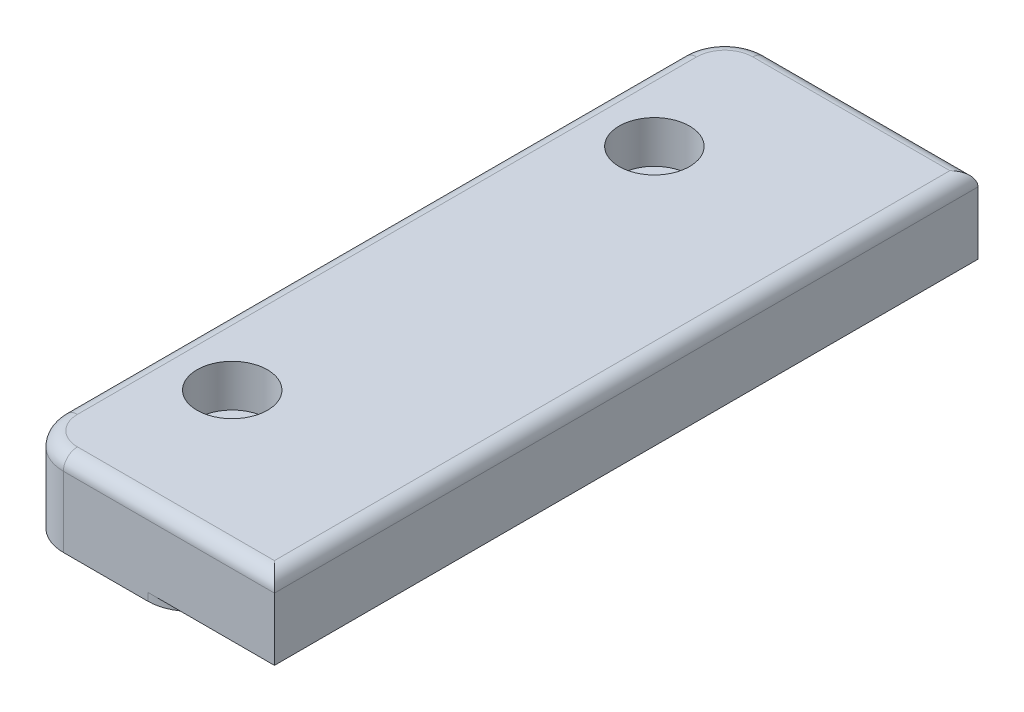
from build123d import *

# Parameters (mm, degrees)
BOSS_EXTRUDE1_DEPTH = 50
FILLET1_R           = 3
SKETCH3_R           = 2.5
CUT_EXTRUDE1_DEPTH  = 3
SKETCH4_R           = 1.5
CUT_EXTRUDE2_DEPTH  = 52.816130281
SKETCH5_R           = 1.5
CUT_EXTRUDE3_DEPTH  = 52.816130281
FILLET5_R           = 3
FILLET6_R           = 3
FILLET7_R           = 1


with BuildPart() as part:
    # Sketch1 → Boss-Extrude1 (new body)
    with BuildSketch(Plane.XY):
        Polygon((-4.736842105, 0), (-4.736842105, 6), (13.263157895, 6), (13.263157895, 0.55), (7.263157895, 0.55), (7.263157895, 0), align=None)
    extrude(amount=BOSS_EXTRUDE1_DEPTH)

    # Fillet1
    fillet1_edges = [part.edges().sort_by_distance(p)[0] for p in [
        (7.263157895, 0.275, 50),
    ]]
    fillet(fillet1_edges, radius=FILLET1_R)

    # Sketch3 → Cut-Extrude1 (cut)
    with BuildSketch(Plane(origin=(0, 6, 0), x_dir=(1, 0, 0), z_dir=(0, 1, 0))):
        with Locations(Location((0.263157895, -10, 0), (0, 0, 180))):
            Circle(SKETCH3_R)
        with Locations(Location((0.263157895, -40, 0), (0, 0, 180))):
            Circle(SKETCH3_R)
    extrude(amount=-CUT_EXTRUDE1_DEPTH, mode=Mode.SUBTRACT)

    # Sketch4 → Cut-Extrude2 (cut, through all)
    with BuildSketch(Plane(origin=(0, 3, 0), x_dir=(1, 0, 0), z_dir=(0, 1, 0))):
        with Locations(Location((0.263157895, -40, 0), (0, 0, 180))):
            Circle(SKETCH4_R)
    extrude(amount=-CUT_EXTRUDE2_DEPTH, mode=Mode.SUBTRACT)

    # Sketch5 → Cut-Extrude3 (cut, through all)
    with BuildSketch(Plane(origin=(0, 3, 0), x_dir=(1, 0, 0), z_dir=(0, 1, 0))):
        with Locations(Location((0.263157895, -10, 0), (0, 0, 180))):
            Circle(SKETCH5_R)
    extrude(amount=-CUT_EXTRUDE3_DEPTH, mode=Mode.SUBTRACT)

    # Fillet5
    fillet5_edges = [part.edges().sort_by_distance(p)[0] for p in [
        (7.263157895, 0.275, 0),
    ]]
    fillet(fillet5_edges, radius=FILLET5_R)

    # Fillet6
    fillet6_edges = [part.edges().sort_by_distance(p)[0] for p in [
        (-4.736842105, 3, 50),
        (-4.736842105, 3, 0),
    ]]
    fillet(fillet6_edges, radius=FILLET6_R)

    # Fillet7
    fillet7_edges = [part.edges().sort_by_distance(p)[0] for p in [
        (13.263157895, 6, 25),
        (5.763157895, 6, 50),
        (-4.736842105, 6, 25),
        (-3.858162449, 6, 49.121320344),
        (-3.858162449, 6, 0.878679656),
        (5.763157895, 6, 0),
    ]]
    fillet(fillet7_edges, radius=FILLET7_R)


solid = part.part
